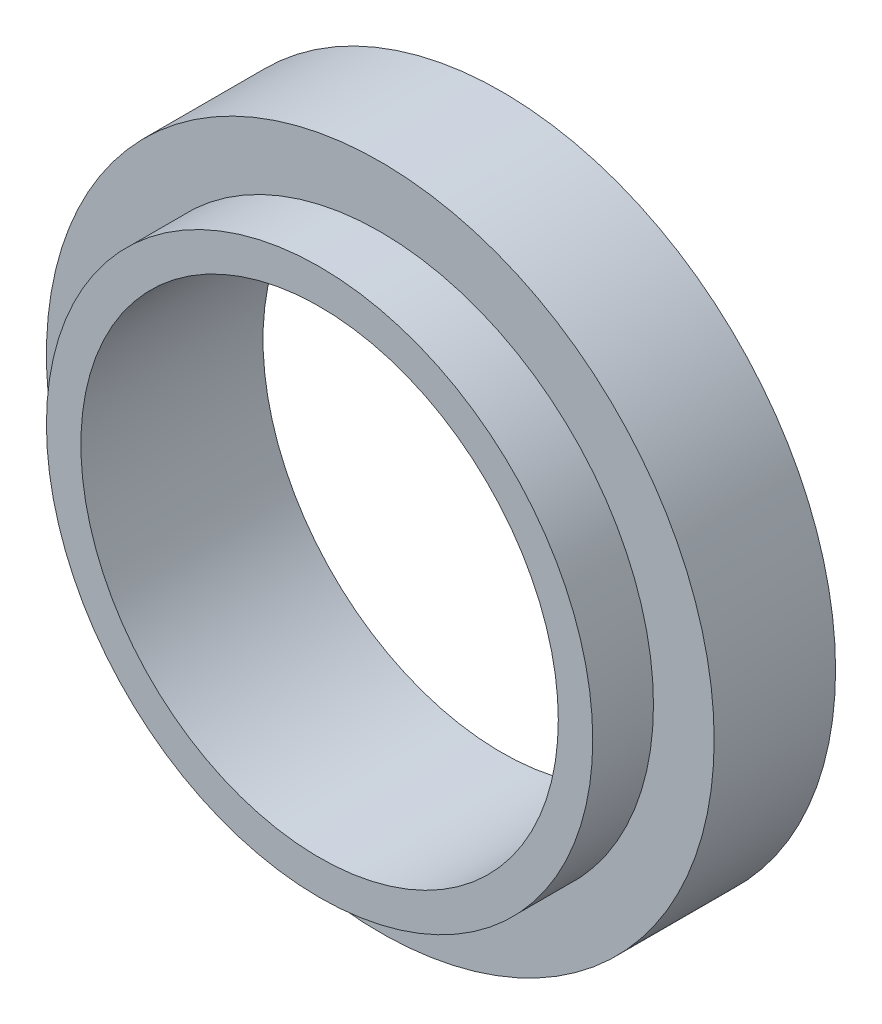
SolidWorks part; units mm, degrees
ref_plane "Front Plane" through (0, 0, 0) normal (0, 0, 1) x (1, 0, 0)
ref_plane "Top Plane" through (0, 0, 0) normal (0, 1, 0) x (1, 0, 0)
ref_plane "Right Plane" through (0, 0, 0) normal (1, 0, 0) x (0, 0, -1)
sketch "Sketch1" plane through (0, 0, 0) normal (0, 0, 1) x (1, 0, 0)
  circle A0 centre (0, 0) radius 27.5
  circle A1 centre (0, 0) radius 19.6623
extrude "Boss-Extrude1" add sketch "Sketch1" along normal blind 10
sketch "Sketch2" plane through (0, 0, 10) normal (0, 0, 1) x (1, 0, 0)
  circle A0 centre (0, 0) radius 22.5
  circle A1 centre (0, 0) radius 19.6623
extrude "Boss-Extrude2" add sketch "Sketch2" along normal blind 5
